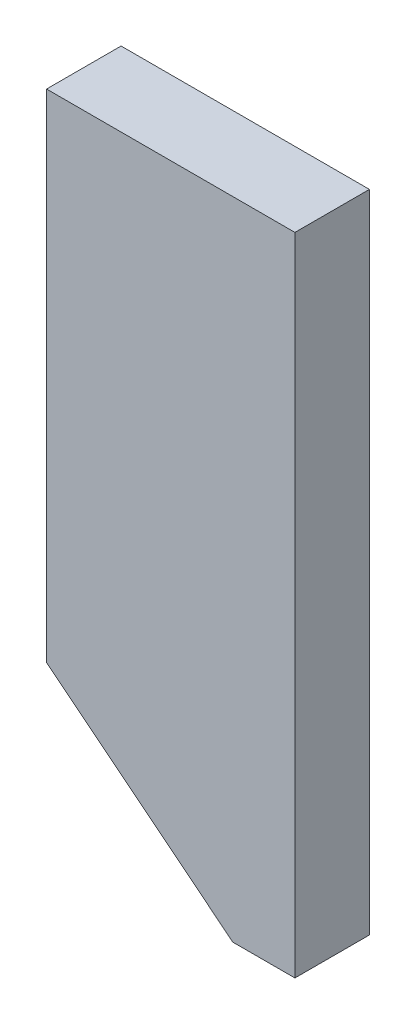
SolidWorks part; units mm, degrees
material "普通碳钢"
ref_plane "Front Plane" through (0, 0, 0) normal (0, 0, 1) x (1, 0, 0)
ref_plane "Top Plane" through (0, 0, 0) normal (0, 1, 0) x (1, 0, 0)
ref_plane "Right Plane" through (0, 0, 0) normal (1, 0, 0) x (0, 0, -1)
sketch "Sketch1" plane through (0, 0, 0) normal (0, 0, 1) x (1, 0, 0)
  line L0 (-12.5, 155) -> (-12.5, -155)
  line L1 (-12.5, -155) -> (12.5, -155)
  line L2 (12.5, -155) -> (12.5, 155)
  line L3 (12.5, 155) -> (-12.5, 155)
  point P2 (-12.5, 0)
  point P5 (0, 155)
  dimension "D1" = 25
  dimension "D2" = 310
extrude "Extrude1" add sketch "Sketch1" along normal mid plane 12
sketch "Sketch3" plane through (0, 0, 0) normal (0, 0, 1) x (1, 0, 0)
  line L0 (0, 0) -> (-156.1525, 0) construction
  line L1 (-12.5, 155) -> (-72.5, 155)
  line L2 (-72.5, 155) -> (-102.5, 131)
  line L3 (-102.5, 131) -> (-102.5, 51)
  line L4 (-102.5, 51) -> (-12.5, 51)
  line L5 (-12.5, 155) -> (-12.5, -155) construction
  line L6 (-12.5, 51) -> (-12.5, 155)
  line L7 (-12.5, -51) -> (-12.5, -155)
  line L8 (-102.5, -51) -> (-12.5, -51)
  line L9 (-102.5, -131) -> (-102.5, -51)
  line L10 (-72.5, -155) -> (-102.5, -131)
  line L11 (-12.5, -155) -> (-72.5, -155)
  dimension "D1" = 51
  dimension "D2" = 90
  dimension "D3" = 60
  dimension "D4" = 80
extrude "Extrude3" add sketch "Sketch3" along normal mid plane 12
sketch "Sketch4" plane through (0, 0, 6) normal (0, 0, 1) x (1, 0, 0)
  line L1 (-102.5, -51) -> (-62.5, -51)
  line L2 (-102.5, -51) -> (-102.5, -179.0827)
  line L3 (-102.5, -179.0827) -> (-62.5, -179.0827)
  line L4 (-62.5, -51) -> (-62.5, -179.0827)
  dimension "D1" = 40
extrude "Cut-Extrude1" cut sketch "Sketch4" against normal blind 22 flip side to cut
